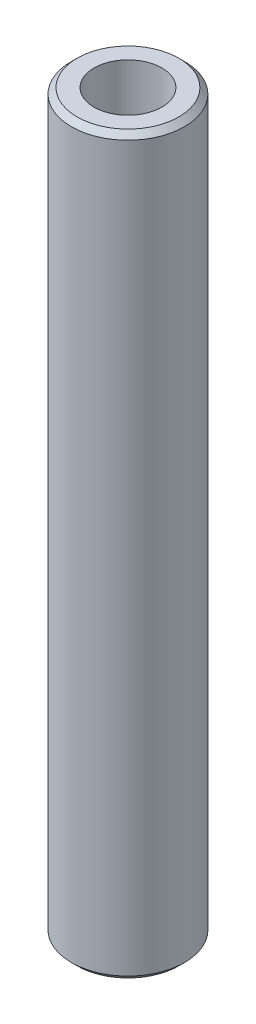
from build123d import *

# Parameters (mm, degrees)
SKETCH1_R           = 5
BOSS_EXTRUDE1_DEPTH = 65
CHAMFER1_SIZE       = 0.5


with BuildPart() as part:
    # Sketch1 → Boss-Extrude1 (new body)
    with BuildSketch(Plane(origin=(0, 0, 0), x_dir=(1, 0, 0), z_dir=(0, 1, 0))):
        with Locations(Location((0, 0, 0), (0, 0, 270))):
            Circle(SKETCH1_R)
    extrude(amount=BOSS_EXTRUDE1_DEPTH)

    # Sketch2 → Ø18.0 (18) Diameter Hole1 (revolve, cut)
    with BuildSketch(Plane(origin=(0, 65, 0), x_dir=(0, 0, 1), z_dir=(1, 0, 0))):
        Polygon((0, 0), (0, 11.802581857), (3, 10), (3, 0), align=None)
    f_18_0_18_diameter_hole1 = revolve(axis=Axis((0, 71.35, 0), (0, -1, 0)), mode=Mode.SUBTRACT)

    # Mirror1: Ø18.0 (18) Diameter Hole1 across plane
    add(f_18_0_18_diameter_hole1.mirror(Plane.ZX.offset(32.5)), mode=Mode.SUBTRACT)

    # Chamfer1
    chamfer1_edges = [part.edges().sort_by_distance(p)[0] for p in [
        (0, 0, -5),
        (0, 65, -5),
    ]]
    chamfer(chamfer1_edges, length=CHAMFER1_SIZE)


solid = part.part
